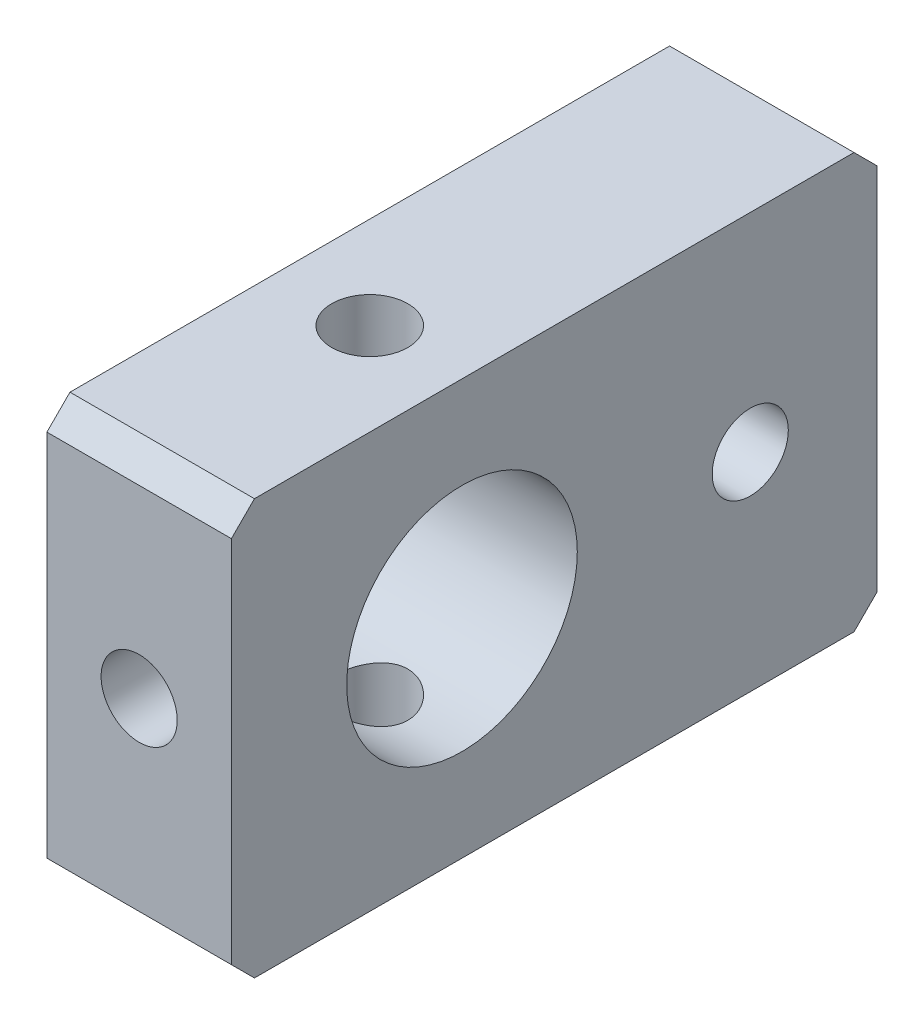
from build123d import *

# Parameters (mm, degrees)
SKETCH_1_W              = 28
SKETCH_1_H              = 18
EXTRUDE_1_DEPTH         = 4
SKETCH_2_R              = 5
CUT_EXTRUDE_1_DEPTH     = 19.466185313
HOLE_WIZARD_M4_1_REACH  = 31.682
HOLE_WIZARD_M4_1_BORE_R = 1.65
HOLE_WIZARD_M4_2_D      = 3.3
HOLE_WIZARD_M4_3_D      = 3.3
CHAMFER_1_SIZE          = 1


with BuildPart() as part:
    # 草图1 → 凸台-拉伸1 (new, symmetric)
    with BuildSketch(Plane(origin=(0, 0, 0), x_dir=(0, 0, -1), z_dir=(1, 0, 0))):
        Rectangle(SKETCH_1_W, SKETCH_1_H)
    extrude(amount=EXTRUDE_1_DEPTH, both=True)

    # 草图2 → 切除-拉伸1 (cut, through all)
    with BuildSketch(Plane(origin=(4, 0, 0), x_dir=(0, 0, -1), z_dir=(1, 0, 0))):
        with Locations((-4, 0)):
            Circle(SKETCH_2_R)
    extrude(amount=-CUT_EXTRUDE_1_DEPTH, mode=Mode.SUBTRACT)

    # M4 螺纹孔1 bore → M4 螺纹孔1 (cut, up to next)
    with BuildSketch(Plane.XY.offset(14), mode=Mode.PRIVATE) as hole_wizard_m4_1_sk1:
        Circle(HOLE_WIZARD_M4_1_BORE_R)
    hole_wizard_m4_1_tool1 = extrude(hole_wizard_m4_1_sk1.sketch, amount=-HOLE_WIZARD_M4_1_REACH, mode=Mode.PRIVATE) & part.part
    add(hole_wizard_m4_1_tool1.solids().sort_by_distance((0, 0, 14))[0], mode=Mode.SUBTRACT)

    # M4 螺纹孔2 (through all)
    with Locations(Plane(origin=(4, 0, 0), x_dir=(0, 0, -1), z_dir=(1, 0, 0))):
        with Locations((8.5, 0)):
            Hole(HOLE_WIZARD_M4_2_D / 2)

    # M4 螺纹孔3 (through all)
    with Locations(Plane(origin=(0, 9, 0), x_dir=(1, 0, 0), z_dir=(0, 1, 0))):
        with Locations((0, -4)):
            Hole(HOLE_WIZARD_M4_3_D / 2)

    # 倒角1
    chamfer_1_edges = [part.edges().sort_by_distance(p)[0] for p in [
        (0, 9, 14),
        (0, 9, -14),
        (0, -9, -14),
        (0, -9, 14),
    ]]
    chamfer(chamfer_1_edges, length=CHAMFER_1_SIZE)


solid = part.part
